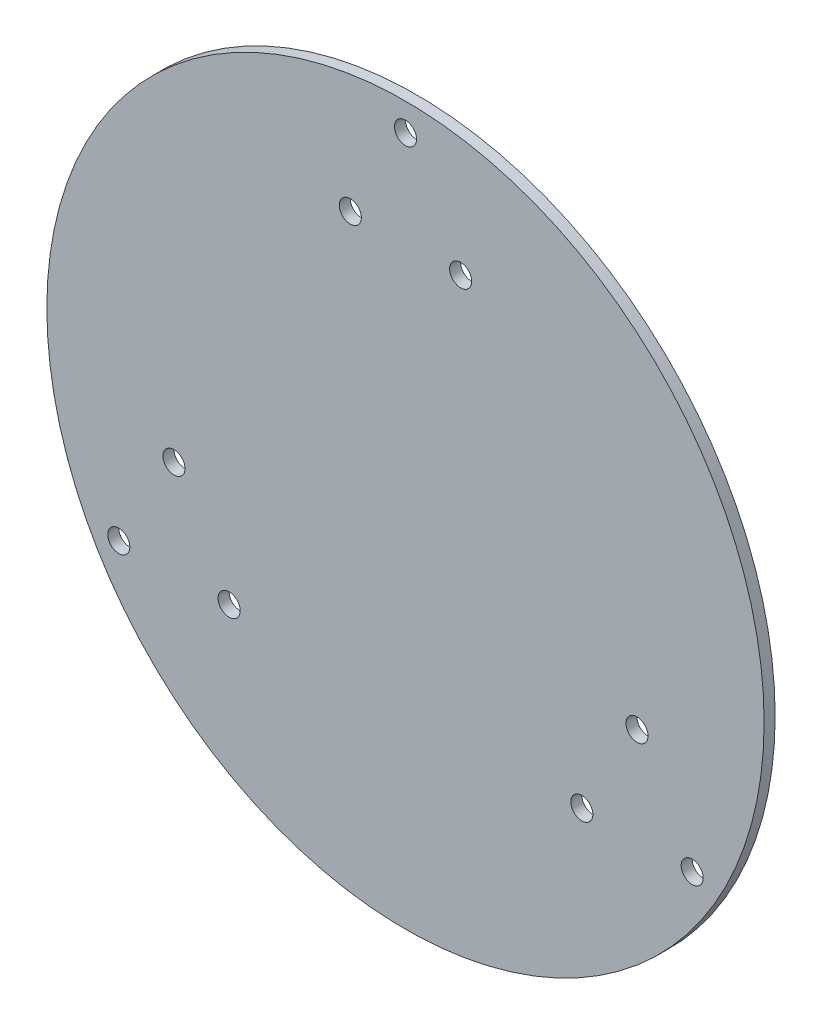
from build123d import *

# Parameters (mm, degrees)
SKETCH1_R           = 65
BOSS_EXTRUDE1_DEPTH = 2
SKETCH3_R           = 2
CUT_EXTRUDE1_DEPTH  = 92.945636112


with BuildPart() as part:
    # Sketch1 → Boss-Extrude1 (new body)
    with BuildSketch(Plane.XY):
        Circle(SKETCH1_R)
    extrude(amount=BOSS_EXTRUDE1_DEPTH)

    # Sketch3 → Cut-Extrude1 (cut, through all)
    with BuildSketch(Plane.XY.offset(2)):
        with Locations((0, 60)):
            Circle(SKETCH3_R)
        with Locations((10, 42.679491924)):
            Circle(SKETCH3_R)
        with Locations((-10, 42.679491924)):
            Circle(SKETCH3_R)
        with Locations((31.961524227, -30)):
            Circle(SKETCH3_R)
        with Locations((41.961524227, -12.679491924)):
            Circle(SKETCH3_R)
        with Locations((51.961524227, -30)):
            Circle(SKETCH3_R)
        with Locations((-41.961524227, -12.679491924)):
            Circle(SKETCH3_R)
        with Locations((-31.961524227, -30)):
            Circle(SKETCH3_R)
        with Locations((-51.961524227, -30)):
            Circle(SKETCH3_R)
    extrude(amount=-CUT_EXTRUDE1_DEPTH, mode=Mode.SUBTRACT)


solid = part.part
